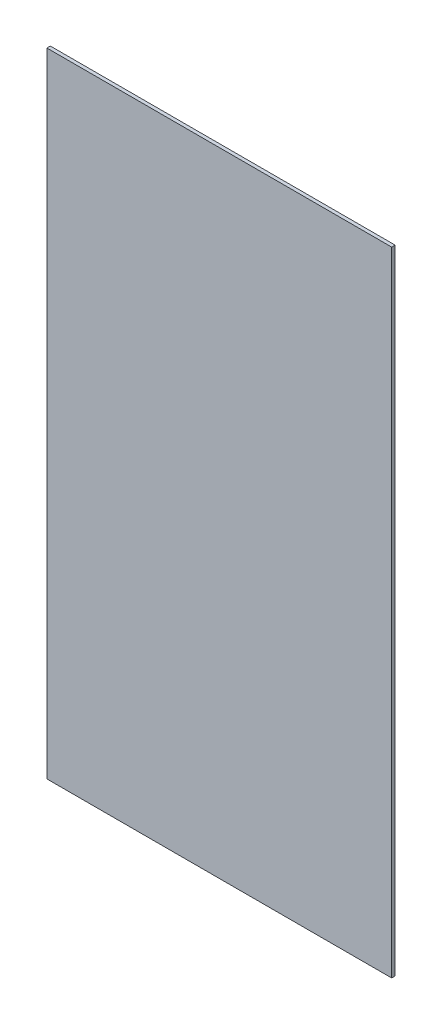
from build123d import *

# Parameters (mm, degrees)
SKETCH_1_W      = 499
SKETCH_1_H      = 916
EXTRUDE_1_DEPTH = 5


with BuildPart() as part:
    # 草图1 → 凸台-拉伸1 (new body)
    with BuildSketch(Plane.XY):
        Rectangle(SKETCH_1_W, SKETCH_1_H)
    extrude(amount=EXTRUDE_1_DEPTH)


solid = part.part
